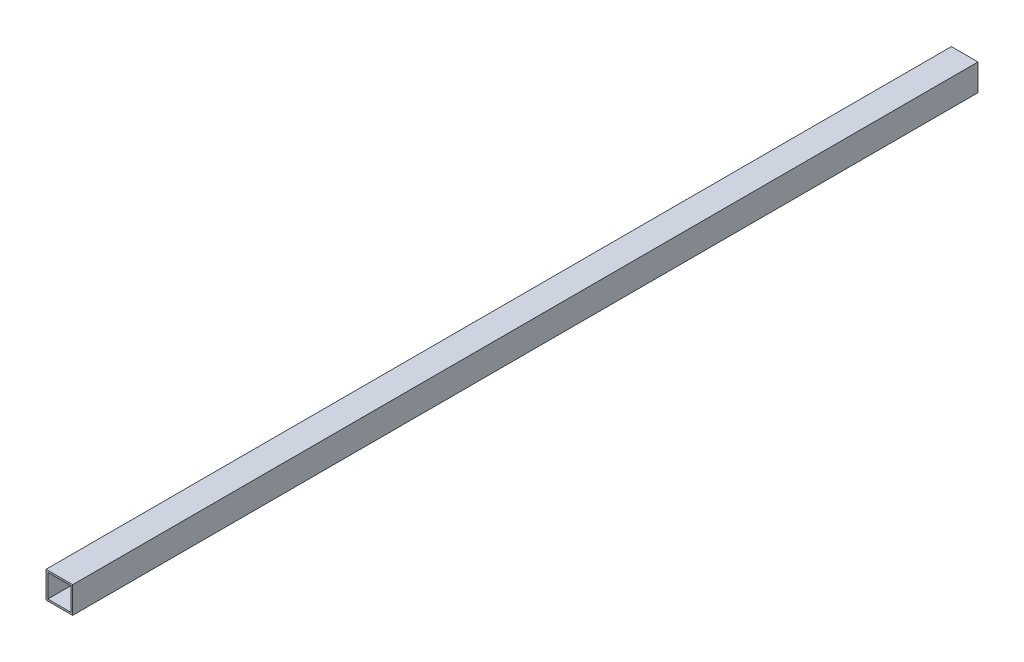
SolidWorks part; units mm, degrees
ref_plane "前视基准面" through (0, 0, 0) normal (0, 0, 1) x (1, 0, 0)
ref_plane "上视基准面" through (0, 0, 0) normal (0, 1, 0) x (1, 0, 0)
ref_plane "右视基准面" through (0, 0, 0) normal (1, 0, 0) x (0, 0, -1)
sketch "草图1" plane through (0, 0, 0) normal (0, 0, 1) x (1, 0, 0)
  line L0 (13, 13) -> (-13, 13)
  line L1 (15, -15) -> (-15, -15)
  line L2 (15, -15) -> (15, 15)
  line L3 (15, 15) -> (-15, 15)
  line L4 (-15, -15) -> (-15, 15)
  line L5 (15, -15) -> (-15, 15) construction
  line L6 (15, 15) -> (-15, -15) construction
  line L7 (-13, -13) -> (-13, 13)
  line L8 (13, -13) -> (-13, -13)
  line L9 (13, -13) -> (13, 13)
  point P0 (0, 0)
  dimension "D1" = 30
  dimension "D2" = 2
extrude "凸台-拉伸1" add sketch "草图1" along normal mid plane 1020
sketch "草图2" plane through (0, 0, 510) normal (0, 0, 1) x (1, 0, 0)
  circle A1 centre (0, 0) radius 2.3345
